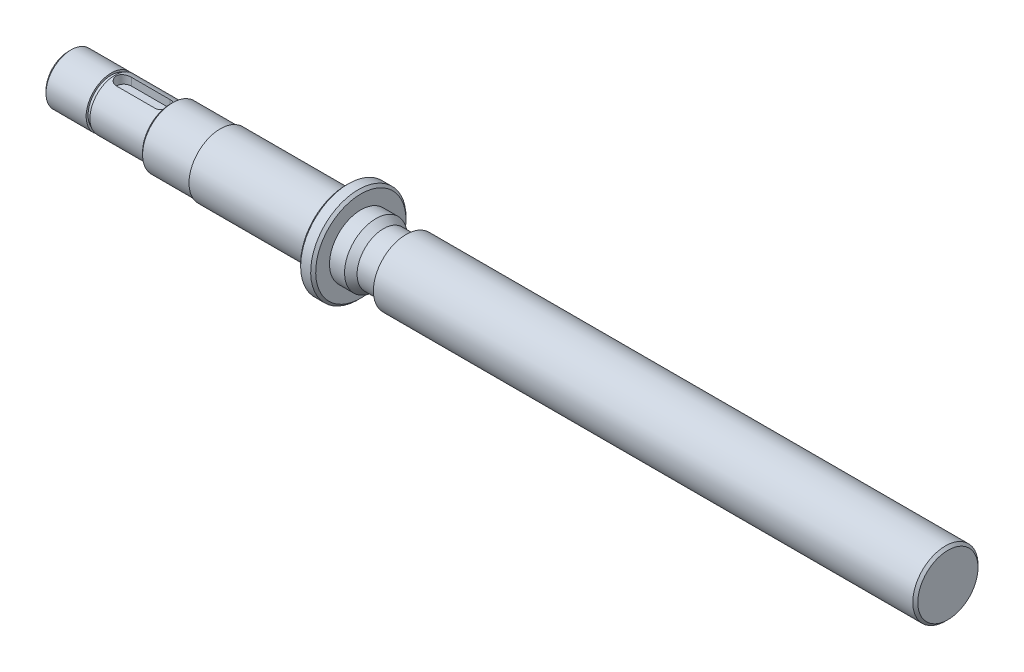
from build123d import *

# Parameters (mm, degrees)
CUT_EXTRUDE_3_DEPTH = 352.939625504
CHAMFER_1_SIZE      = 1


with BuildPart() as part:
    # 草图1 → 旋转1 (revolve)
    with BuildSketch(Plane.XY):
        Polygon((0, 0), (0, 10), (17, 10), (17, 9.25), (18.5, 9.25), (18.5, 10), (40.5, 10), (40.5, 12), (60.5, 12), (60.5, 12.5), (110.5, 12.5), (110.5, 19), (116.5, 19), (116.5, 12.5), (122.5, 12.5), (125.5, 10.5), (134.5, 10.5), (134.5, 13), (350.5, 13), (350.5, 0), align=None)
    revolve(axis=Axis((350.5, 0, 0), (-1, 0, 0)))

    # 草图2 → 切除-拉伸3 (cut, through all)
    with BuildSketch(Plane(origin=(0, 6.5, 0), x_dir=(1, 0, 0), z_dir=(0, 1, 0))):
        with BuildLine():
            Line((22, 3), (37.5, 3))
            ThreePointArc((37.5, 3), (40.5, 0), (37.5, -3))
            Line((37.5, -3), (22, -3))
            ThreePointArc((22, -3), (19, 0), (22, 3))
        make_face()
    extrude(amount=CUT_EXTRUDE_3_DEPTH, mode=Mode.SUBTRACT)

    # 倒角1
    chamfer_1_edges = [part.edges().sort_by_distance(p)[0] for p in [
        (350.5, -13, 0),
        (116.5, -19, 0),
        (110.5, -19, 0),
        (40.5, -12, 0),
        (0, -10, 0),
    ]]
    chamfer(chamfer_1_edges, length=CHAMFER_1_SIZE)


solid = part.part
